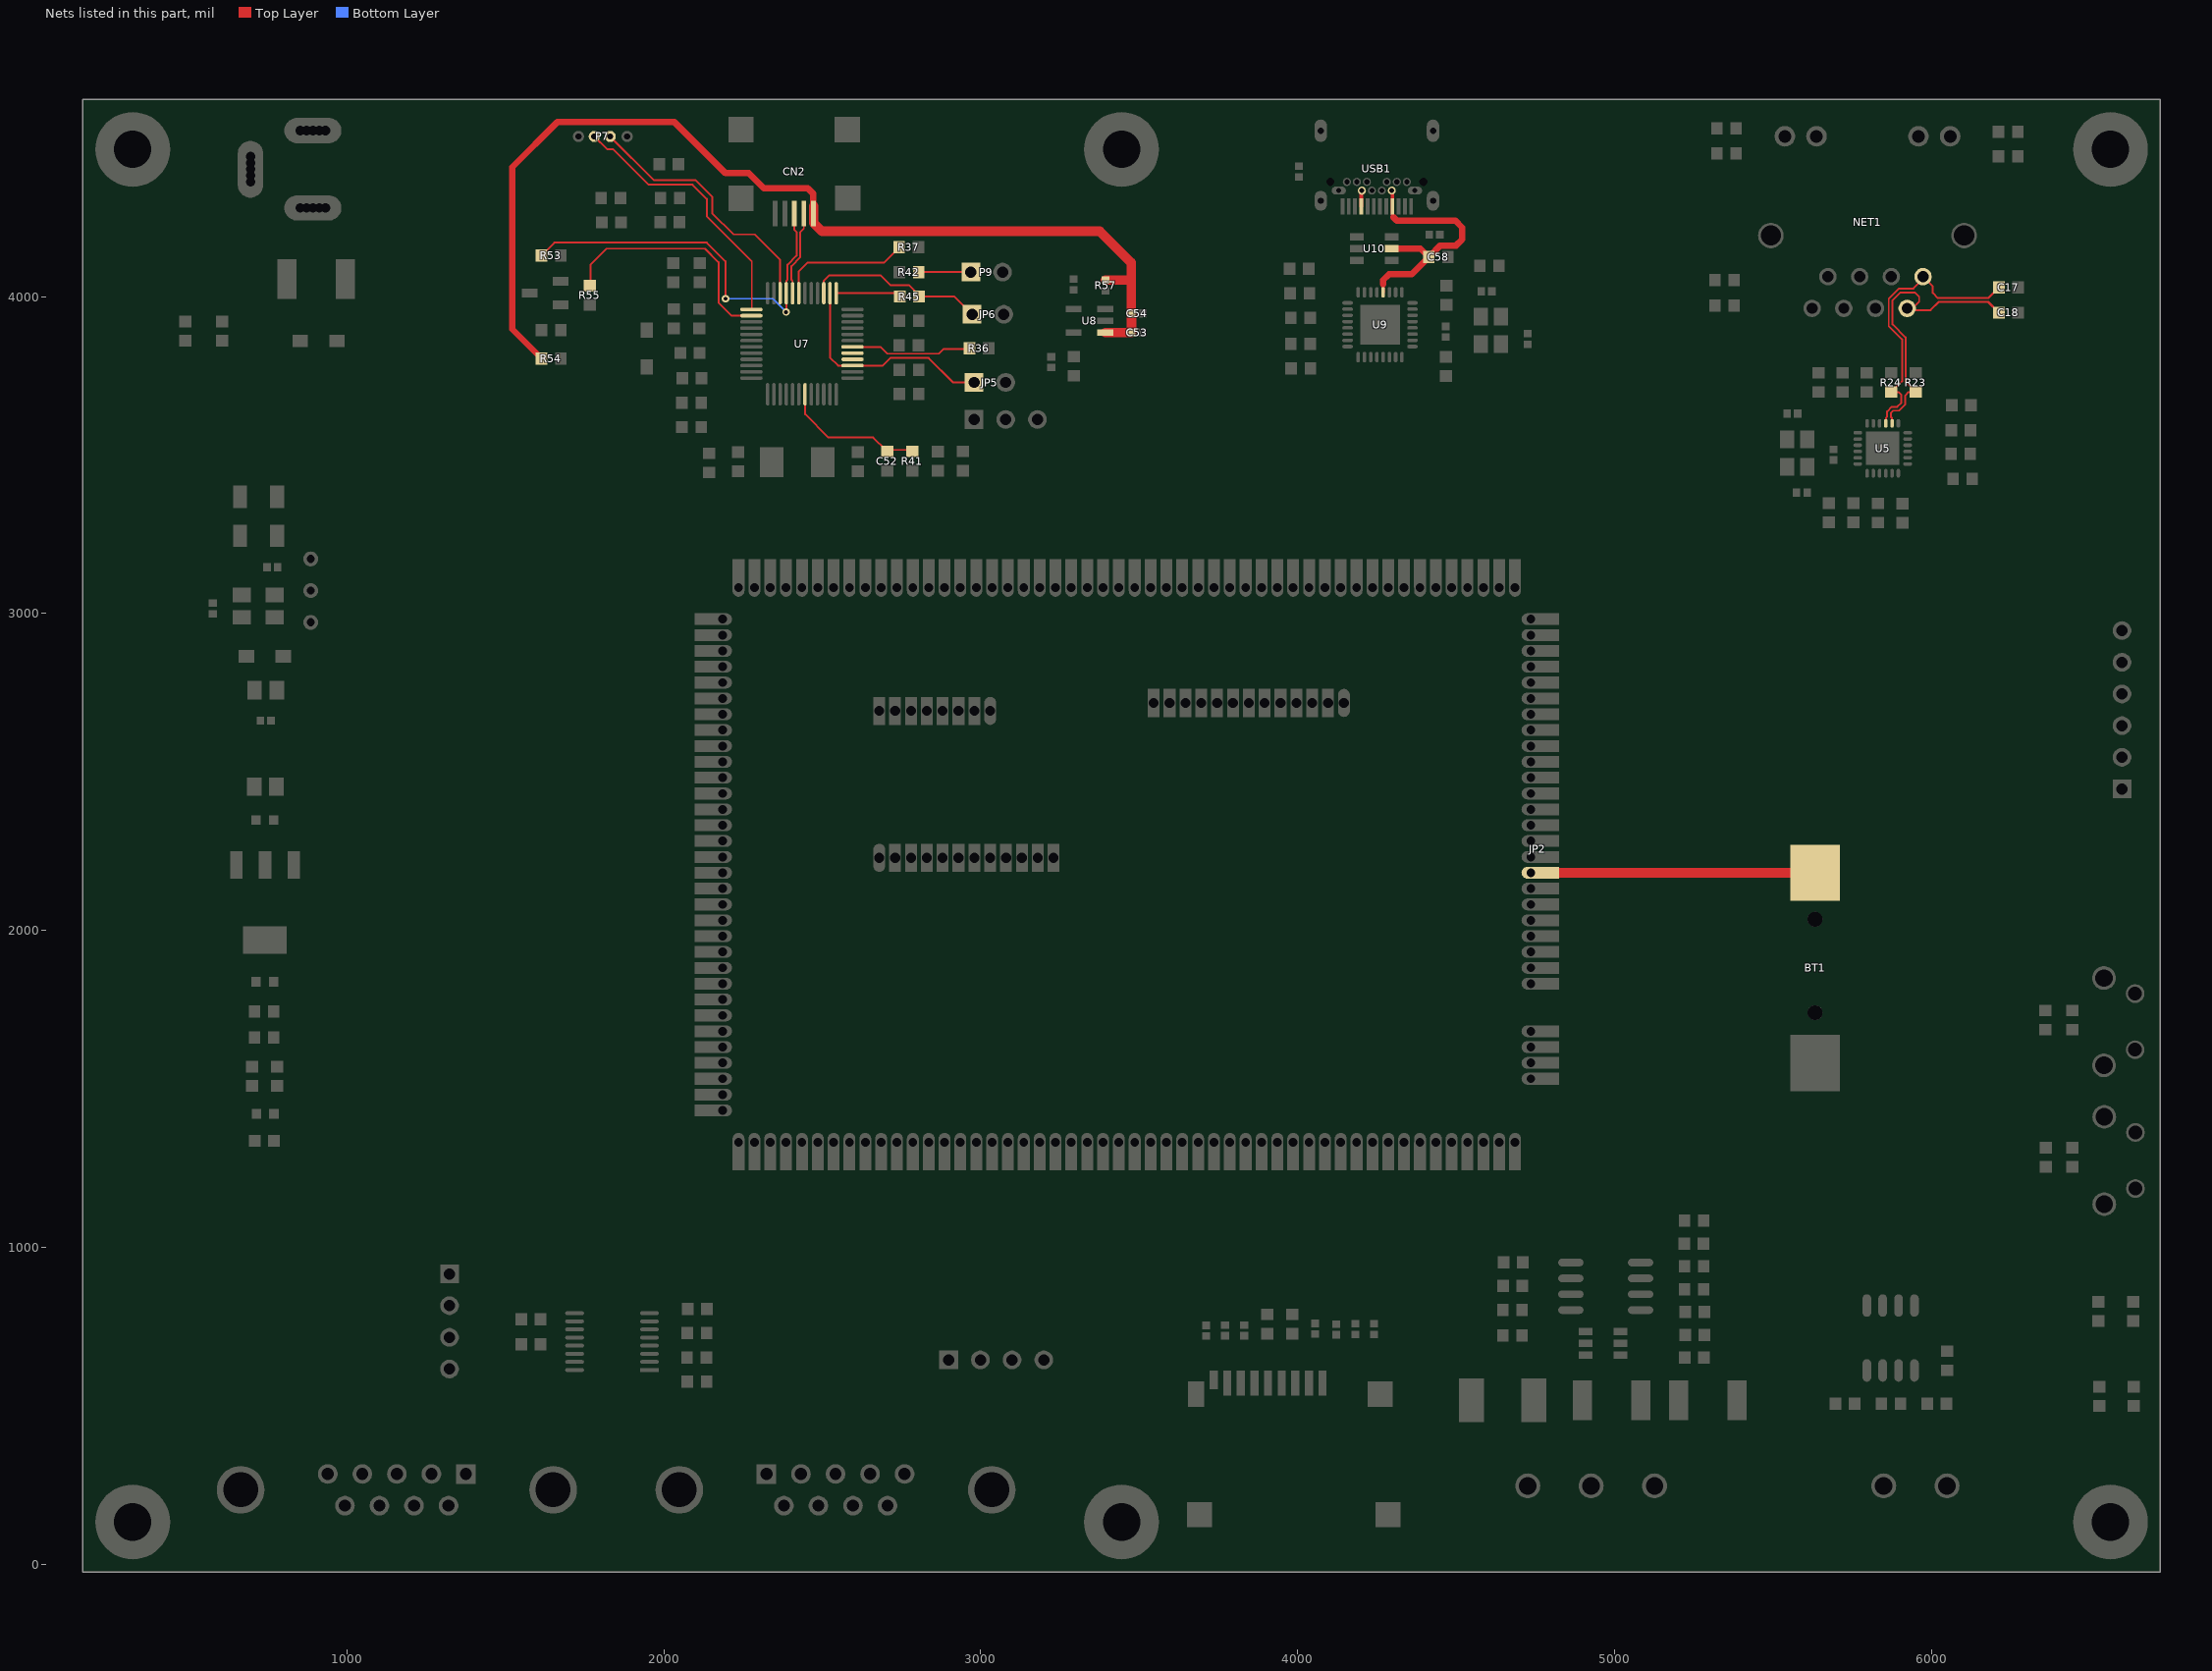
[diagram p0: the nets of this part, all layers, seen from the top]
# Altium PCB MISC105202-15.PcbDoc (part 4 of 4)
Units mil, origin at the board's own origin, x right, y up, seen from the top; angles counter-clockwise.
Board outline 6555.12 x 4645.67 mil, 2 copper layers (Top Layer, Bottom Layer); 182 components, 258 nets, 994 pads, 145 vias.
Unrouted connection lines stored in the file: 1.

## Via types
v1: diameter 24, hole 12, Top Layer to Bottom Layer, 128 vias
v2: diameter 19.68, hole 7.87, Top Layer to Bottom Layer, 9 vias
v3: diameter 50, hole 50, Top Layer to Bottom Layer, 4 vias
v4: diameter 30, hole 15, Top Layer to Bottom Layer, 2 vias
v5: diameter 137.8, hole 137.8, Top Layer to Bottom Layer, 2 vias

## Nets (pads, with @x,y where several pads share a name; then routed paths per layer and width w, separated by ;. In a path a pad name is that pad's centre, name@x,y a point inside that pad or via, vN(x,y) a via of type N, cw(c..) or ccw(c..) an arc to the next point about the centre after c; other vN are vias at no path point) (continued)
STLINK_U5V: C53.1 C54.2 CN2.1 R54.2 R57.2 U8.1 | length 3297.5
  Top Layer w20: R54.2@1610,3807 1610,3809 1522,3897 1522,4408 1664,4550 2034,4550 2195,4389 2269,4389 2317,4341 2455,4341 2472,4324 CN2.1@2472,4261.54
  Top Layer w30: CN2.1@2473,4285 2473,4232 2499,4206 3376,4206 3475,4107 C54.2@3475,3943 ; U8.1@3393,3886.2 3475.8,3886.2 3476,3886 C54.2@3476,3947 ; R57.2@3394,4051.73 3473.27,4051.73 3474,4051
STLINK_USB_DM: CN2.2 U7.32 | length 269
  Top Layer w6: U7.32@2406.47,4010.45 2406.47,4049 2402.63,4052.84 2402.63,4095.63 2431,4124 2431,4203 2442,4214 CN2.2@2442,4261.54
STLINK_USB_DP: CN2.3 R53.1 U7.33 | length 1268.3
  Top Layer w6: R53.1@1614.69,4130 1654.69,4170 2136,4170 2195,4111 v1(2195,3993) ; v1@2386.79,3957.21 U7.33@2386.79,4010.45 2386.79,4049 2390.63,4052.84 2390.63,4100.6 2419,4128.97 2419,4203 2412,4210 CN2.3@2412,4261.54
  Bottom Layer w6: v1(2195,3993) 2344,3993 v1(2386,3951)
STLK_MCO: P9.1 R42.2 | length 152.7
  Top Layer w6: R42.2@2804.32,4077 P9.1@2957,4077
STM_JTCK: P7.2 U7.37 | length 841.4
  Top Layer w6: P7.2@1781,4505 1821,4465 1840,4465 1952,4353 2091,4353 2136,4308 2136,4253 2278,4111 U7.37@2278,3962
STM_JTMS: P7.3 U7.34 | length 834.2
  Top Layer w6: P7.3@1829,4505 P7.3@1829,4506 ; P7.3@1831,4505 1969,4367 2101,4367 2153,4315 2153,4263 2220,4196 2287,4196 2367.1,4115.9 U7.34@2367.1,4010.45
STM_RST: C52.2 R41.1 U7.7 | length 449.4
  Top Layer w6: U7.7@2445.84,3674 U7.7@2445.84,3691.55 ; U7.7@2446,3674 2446,3629 2520,3555 2661,3555 2700,3516 2779,3516 R41.1@2784,3511
T_JTCK: JP5.1 U7.15 U7.26 | length 687.8
  Top Layer w6: U7.26@2524.58,4010.45 2524.58,3807.42 2550,3782 U7.15@2583,3782 ; U7.15@2605,3782 2691,3782 2715,3806 2836,3806 2913,3729 JP5.1@2979,3729
T_JTDI: U7.17
T_JTDO: U7.16
T_JTMS: JP6.1 R45.2 U7.27 | length 524.2
  Top Layer w6: U7.27@2504.9,4010.45 2504.9,4049.9 2521,4066 2685,4066 2715,4036 2774,4036 R45.2@2799,4011 ; R45.2@2805.32,4000 2917,4000 JP6.1@2952,3965
T_NRST: R36.1 U7.18 | length 381.8
  Top Layer w6: U7.18@2595.45,3841.16 2683.84,3841.16 2705.29,3819.71 2868.71,3819.71 2884,3835 R36.1@2962,3835
T_SWDIO_IN: R45.1 U7.25 | length 192.4
  Top Layer w6: U7.25@2544.27,4010.45 2734.45,4010.45 R45.1@2736,4012
T_SWO: R37.1 U7.31 | length 405.2
  Top Layer w6: U7.31@2426.16,4010.45 2426.16,4079.16 2454,4107 2696,4107 R37.1@2735,4146
TD_N: C18.1 NET1.2 R23.1 U5.20 | length 929.9
  Top Layer w6: U5.20@5875.53,3599.74 5875.53,3617 5874.69,3617 5871.69,3620 5871.69,3632 5879.69,3640 5896.97,3640 5917,3660.03 5917,3688 5927.69,3698.69 R23.1@5950,3698.69 5918,3730.69 5918,3870.97 5877,3911.97 5877,3988 5902,4013 5947,4013 5961,3999 5961,3984 NET1.2@5942,3965 ; NET1.2@5928,3962 5933,3957 5997,3957 6023,3983 6178.68,3983 C18.1@6212.68,3949
TD_P: C17.1 NET1.1 R24.1 U5.21 | length 906.2
  Top Layer w6: U5.21@5855.84,3599.74 5855.84,3617 5859.69,3620.84 5859.69,3636.97 5874.71,3652 5892,3652 5905,3665 5905,3689 5895.31,3698.69 R24.1@5873,3698.69 5907,3732.69 5907,3865 5865,3907 5865,3992.97 5897.03,4025 5943,4025 NET1.1@5971,4053 ; NET1.1@5973.2,4062.63 6004,4031.83 6004,4011 6020,3995 6178.68,3995 C17.1@6212.68,4029
USB_RENUMN: R55.2 U7.38 | length 756.2
  Top Layer w6: R55.2@1769.5,4039.5 1769.5,4101.5 1819,4151 2130,4151 2173,4108 2173,3981 2214.42,3939.58 U7.38@2276.55,3939.58
  Top Layer w10: R55.2@1767,4034.32 R55.2@1767,4039
VBAT: BT1.1 JP2.16 | length 843.4
  Top Layer w30: JP2.16@4780.49,2181.87 5620.87,2181.87 BT1.1@5623,2184
VBUS: C58.2 U9.4 U10.5 USB1.A4 USB1.A9 USB1.B4 USB1.B9 | length 831.8
  Top Layer w10: U9.4@4269.84,4013.36 4269.84,4038.84
  Top Layer w12: USB1.B4@4200,4328 4200.79,4327.21 USB1.A9@4200.79,4284.95 ; 4299.21,4255.79 USB1.A4@4299.21,4284.95 USB1.B9@4299.21,4330.79
  Top Layer w20: 4269.84,4038.84 4269.84,4051.84 4288,4070 4360,4070 C58.2@4406,4116 ; 4301.78,4250.78 4312.56,4240 4497,4240 4519,4218 4519,4180 4500,4161 4450,4161 C58.2@4418,4129 ; U10.5@4309,4151 4387.69,4151 C58.2@4413.69,4125 C58.2@4417.84,4129.16
pads on no net: BT1.0 J1. J1.1 J1.4 J1.6 J1.7 J1.8 J1.9 J2. J2.1 J2.4 J2.6 J2.7 J2.8 J2.9 NET1.0 NET1.7 P8.2 S1.0 S2.0 U4.3 U4.4 U4.6 U5.0 U5.10 U7.3 U7.4 U7.11 U7.14 U7.19 U7.22 U7.28 U7.40 U7.41 U7.42 U7.43 U7.45 U7.46 U9.3 U9.5 U9.9 U9.10 U10.3 U10.4 USB1.0 USB1.A2 USB1.A3 USB1.A8 USB1.A10 USB1.A11 USB1.B2 USB1.B3 USB1.B8 USB1.B10 USB1.B11 Y1.2 Y1.4 Y3.2 Y3.4
copper on no net:
  other v3: 3797.69,136.56 4117.69,136.56 2322,4404.63 2504,4406.63
  other v5: 5573,4312.63 6023,4312.63

## Polygon pours and split planes (outlines as drawn)
3V3 on Top Layer "TopLayer-No Net" (solid, remove dead copper, pour order 1003): 712,2235 712,2085 669,2042 665,2038 665,1950 665,1929 679,1915 690,1904 707,1904 739,1904 742,1904 748,1898 753,1893 753,1852 753,1557 759,1551 771,1551 831,1551 842,1562 844,1564 844,1594 844,2044 798,2090 771,2117 771,2176 771,2247 764,2254 762,2256 749,2256 717,2256 712,2251 712,2235
+5V on Top Layer "TopLayer-No Net" (solid, remove dead copper, pour order 1002): 773,2870 773,2847 773,2829 764,2820 754,2810 754,2781 754,2617 754,2320 787,2287 808,2266 808,2246 808,2164 868,2104 1013,1959 1164,1808 1164,1450 1164,935 1190,909 1217,882 1319,882 1358,882 1363,887 1372,896 1372,923 1372,1903 1028,2247 924,2351 924,2655 924,2860 911,2873 893,2891 844,2891 779,2891 773,2885 773,2870
+3V3_ST_LINK on Top Layer "TopLayer-No Net" (solid, remove dead copper, pour order 1001): 2862,3909 2862,3874 2871,3865 2876,3860 2890,3860 2907,3860 2920,3873 2926,3879 2926,3906 2902,3930 2881,3930 2881,3929 2862,3910
+3V3_ST_LINK on Top Layer "TopLayer-No Net" (solid, remove dead copper, pour order 1000): 2758,3450 2758,3374 2766,3366 2772,3360 2787,3360 2798,3360 2808,3370 2816,3378 2816,3412 2816,3458 2803,3471 2793,3471 2766,3471 2759,3464 2757,3462 2757,3449
NetCN1_1 on Top Layer "Top Layer-No Net" (solid, remove dead copper, pour order 1000): 717,4126 717,4011 717,3973 726,3964 733,3957 770,3957 854,3957 860,3963 866,3969 866,4025 866,4163 890,4187 900,4197 935,4197 976,4197 998,4219 1017,4238 1017,4261 1017,4319 1010,4326 990,4346 922,4346 798,4346 780,4328 717,4265 717,4126
NetD6_1 on Top Layer "Top Layer-No Net" (solid, remove dead copper, pour order 1001): 942,3875 942,3835 945,3832 947,3830 955,3822 1041,3822 1068,3822 1077,3831 1080,3834 1080,3889 1080,4121 1073,4128 1016,4128 963,4128 959,4124 956,4121 956,4111 956,3914 947,3905 942,3900 942,3875
AIN2 on Top Layer "Top Layer-No Net" (solid, remove dead copper, pour order 1002): 580,3858 580,3776 585,3771 605,3751 630,3751 678,3751 697,3732 744,3685 744,3413 744,3217 757,3204 769,3192 769,3178 769,3134 771,3132 772,3131 774,3131 906,3131 914,3139 919,3144 919,3177 919,3770 894,3795 881,3808 881,3871 881,3877 875,3883 873,3885 834,3885 587,3885 581,3879 580,3878 580,3858
NetC31_2 on Top Layer "Top Layer-No Net" (solid, remove dead copper, pour order 1003): 551,3002 551,2949 556,2944 561,2939 576,2939 596,2939 601,2934 606,2929 606,2920 606,2851 613,2844 624,2833 649,2833 708,2833 711,2836 712,2837 712,2849 712,2909 720,2917 724,2921 747,2921 901,2921 909,2929 917,2937 917,2968 917,2995 907,3005 901,3011 829,3011 560,3011 551,3002
A3V3 on Top Layer "Top Layer-No Net" (solid, remove dead copper, pour order 1000): 5408,1028 5408,991 5415,984 5420,979 5430,979 5462,979 5471,988 5472,989 5472,1017 5472,1033 5460,1045 5455,1050 5448,1050 5427,1050 5420,1043 5408,1031 5408,1027
3V3 on Top Layer "Top Layer-No Net" (solid, remove dead copper, pour order 1001): 3908,378 3908,342 3915,335 3917,333 3926,333 3966,333 3971,338 3976,343 3976,356 3976,382 3969,389 3965,393 3944,393 3915,393 3911,389 3908,386 3908,378
3V3 on Top Layer "Top Layer-No Net" (solid, remove dead copper, pour order 1002): 3928,224 3928,189 3936,181 3941,176 3957,176 3982,176 3992,186 3995,189 3995,209 3995,224 3988,231 3982,237 3972,237 3941,237 3928,224
3V3 on Top Layer "Top Layer-No Net" (solid, remove dead copper, pour order 1003): 2532,672 2532,638 2532,632 2541,623 2549,615 2570,615 2589,615 2593,619 2597,623 2597,646 2597,662 2585,674 2580,679 2562,679 2539,679 2532,672
3V3 on Top Layer "Top Layer-No Net" (solid, remove dead copper, pour order 1004): 2699,732 2699,714 2699,702 2710,691 2718,683 2729,683 2757,683 2765,691 2767,693 2767,705 2767,722 2757,732 2751,738 2739,738 2705,738 2699,732
AGND on Top Layer "Top Layer-No Net" (solid, remove dead copper, pour order 1005): 5313,335 5313,312 5316,309 5319,306 5327,306 5358,306 5365,313 5368,316 5368,323 5368,340 5365,343 5362,346 5351,346 5317,346 5313,342 5313,335
AGND on Top Layer "Top Layer-No Net" (solid, remove dead copper, pour order 1006): 4620,1017 4620,947 4620,934 4626,928 4633,921 4642,921 4667,921 4671,925 4672,926 4672,940 4672,991 4682,1001 4683,1002 4683,1019 4683,1048 4676,1055 4675,1056 4660,1056 4648,1056 4625,1033 4620,1028 4620,1018
AGND on Top Layer "Top Layer-No Net" (solid, remove dead copper, pour order 1007): 666,1302 666,1240 684,1222 690,1216 710,1216 722,1216 734,1228 747,1241 747,1257 747,1289 734,1302 732,1304 732,1331 732,1355 726,1361 700,1361 681,1361 669,1349 665,1345 665,1302
GND on Top Layer "Top Layer-No Net" (solid, remove dead copper, pour order 1008): -36,4718 -36,-319 32,-251 6917,-251 6917,4633 6832,4718 6815,4735 -19,4735
+3V3_ST_LINK on Bottom Layer "TopLayer-No Net" (solid, remove dead copper, pour order 1006): 2861,3911 2861,3877 2870,3868 2876,3862 2886,3862 2906,3862 2917,3873 2922,3878 2922,3898 2922,3917 2912,3927 2906,3933 2894,3933 2881,3933 2861,3913 2861,3910
+3V3_ST_LINK on Bottom Layer "TopLayer-No Net" (solid, remove dead copper, pour order 1005): 2762,3410 2762,3378 2762,3373 2768,3367 2774,3361 2785,3361 2796,3361 2800,3365 2809,3374 2809,3388 2809,3417 2809,3419 2797,3431 2781,3431 2773,3431 2767,3425 2762,3420 2762,3410
A3V3 on Bottom Layer "Top Layer-No Net" (solid, remove dead copper, pour order 1009): 5407,1023 5407,1000 5407,989 5415,981 5419,977 5436,977 5459,977 5465,983 5470,988 5470,1003 5470,1029 5462,1037 5453,1046 5437,1046 5424,1046 5410,1032 5407,1029 5407,1023
3V3 on Bottom Layer "Top Layer-No Net" (solid, remove dead copper, pour order 1010): 3909,378 3909,232 3909,188 3919,178 3922,175 3942,175 3981,175 3989,183 3992,186 3992,216 3992,375 3977,390 3972,395 3964,395 3926,395 3909,378
3V3 on Bottom Layer "Top Layer-No Net" (solid, remove dead copper, pour order 1011): 2534,668 2534,644 2534,632 2543,623 2553,613 2583,613 2593,613 2609,613 2666,670 2673,677 2705,677 2750,677 2759,686 2768,695 2768,700 2768,728 2758,738 2754,742 2733,742 2665,742 2656,742 2613,699 2595,681 2573,681 2547,681 2534,668
3V3 on Bottom Layer "Top Layer-No Net" (solid, remove dead copper, pour order 1012): 783,1802 783,1782 783,1772 791,1764 805,1750 824,1750 832,1750 839,1757 847,1765 847,1781 847,1818 840,1825 833,1832 826,1832 805,1832 799,1826 783,1810 783,1801
AGND on Bottom Layer "Top Layer-No Net" (solid, remove dead copper, pour order 1013): 5313,341 5313,312 5318,307 5319,306 5329,306 5357,306 5367,316 5368,317 5368,332 5368,336 5358,346 5337,346 5318,346 5313,341
AGND on Bottom Layer "Top Layer-No Net" (solid, remove dead copper, pour order 1014): 4621,1027 4621,1000 4621,996 4626,991 4633,984 4638,984 4669,984 4680,995 4689,1004 4689,1021 4689,1044 4680,1053 4678,1055 4662,1055 4650,1055 4621,1026
AGND on Bottom Layer "Top Layer-No Net" (solid, remove dead copper, pour order 1015): 671,1273 671,1241 689,1223 696,1216 716,1216 721,1216 744,1239 747,1242 747,1256 747,1265 737,1275 724,1288 706,1288 684,1288 677,1281 670,1274 670,1273
GND on Bottom Layer "Top Layer-No Net" (solid, remove dead copper, pour order 1016): 53,4644 53,-183 126,-256 136,-246 7047,-246 7047,4745 6946,4846 6900,4800 602,4800 227,4800 62,4635

## Keep-outs
Keep-Out Layer:
  lines w3.94: 2601.26,2229 3308.74,2229 3308.74,2406.17 2601.26,2406.17 2601.26,2229 ; 2601.26,2515.46 3108.74,2515.46 3108.74,2692.62 2601.26,2692.62 2601.26,2515.46 ; 3467.26,2540.46 4224.74,2540.46 4224.74,2717.62 3467.26,2717.62 3467.26,2540.46
  lines w7.87: 167,-24 167,4621.67 6722.12,4621.67 6722.12,-24 167,-24

## Silkscreen, mask and mechanical layers (free items; w line width, h text height)
Top Overlay:
  lines w6: 2137,1280 2137,3134.33 4786.61,3134.33 4786.61,1280 2137,1280
  lines w7.87: 167,290.96 6722.12,290.96 ; 167,4294.9 6722.12,4294.9
  lines w8: 2186,2181.87 2186.3,2181.57